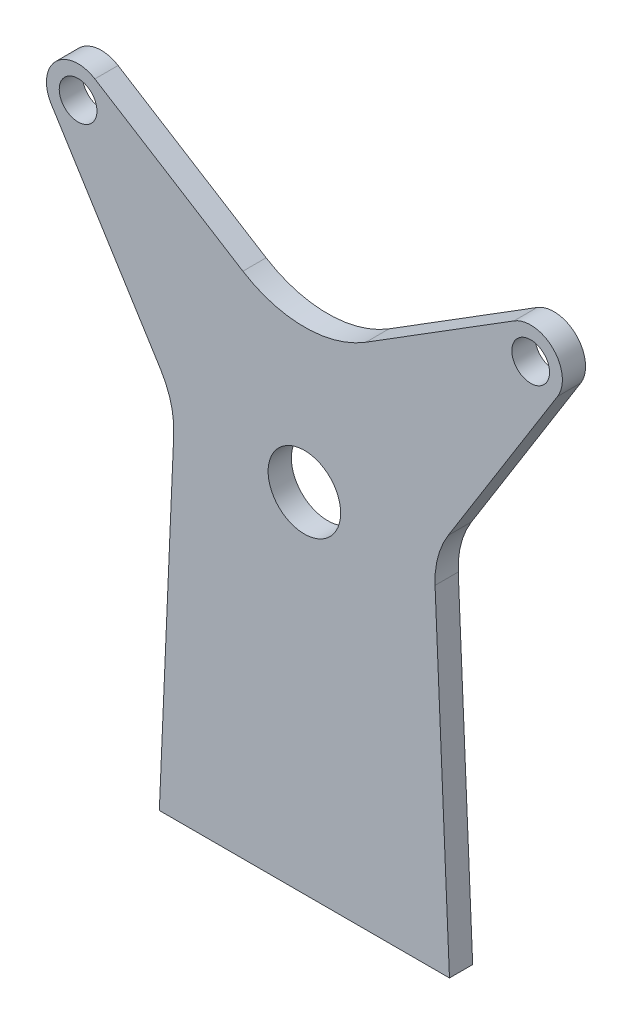
from build123d import *

# Parameters (mm, degrees)
SKETCH1_R           = 12.5
SKETCH1_R_2         = 6.5
BOSS_EXTRUDE1_DEPTH = 4


with BuildPart() as part:
    # Sketch1 → Boss-Extrude1 (new, symmetric)
    with BuildSketch(Plane.XY):
        with BuildLine():
            Line((50, 0), (-50, 0))
            Line((-50, 0), (-45.028143867, 114.700831063))
            ThreePointArc((-45.028143867, 114.700831063), (-45.989821567, 123.642613906), (-49.558557115, 131.897577927))
            Line((-49.558557115, 131.897577927), (-87.251556293, 192.218986015))
            ThreePointArc((-87.251556293, 192.218986015), (-85.713994314, 205.713994314), (-72.218986015, 207.251556293))
            Line((-72.218986015, 207.251556293), (-21.196770569, 175.369337595))
            ThreePointArc((-21.196770569, 175.369337595), (-11.025494233, 170.840793604), (0, 169.291261441))
            ThreePointArc((0, 169.291261441), (11.025494233, 170.840793604), (21.196770569, 175.369337595))
            Line((21.196770569, 175.369337595), (72.218986015, 207.251556293))
            ThreePointArc((72.218986015, 207.251556293), (85.713994314, 205.713994314), (87.251556293, 192.218986015))
            Line((87.251556293, 192.218986015), (49.558557115, 131.897577927))
            ThreePointArc((49.558557115, 131.897577927), (45.989821567, 123.642613906), (45.028143867, 114.700831063))
            Line((45.028143867, 114.700831063), (50, 0))
        make_face()
        with Locations((0, 120)):
            Circle(SKETCH1_R, mode=Mode.SUBTRACT)
        with Locations((78, 198)):
            Circle(SKETCH1_R_2, mode=Mode.SUBTRACT)
        with Locations(Location((-78, 198, 0), (0, 0, 180))):
            Circle(SKETCH1_R_2, mode=Mode.SUBTRACT)
    extrude(amount=BOSS_EXTRUDE1_DEPTH, both=True)


solid = part.part
